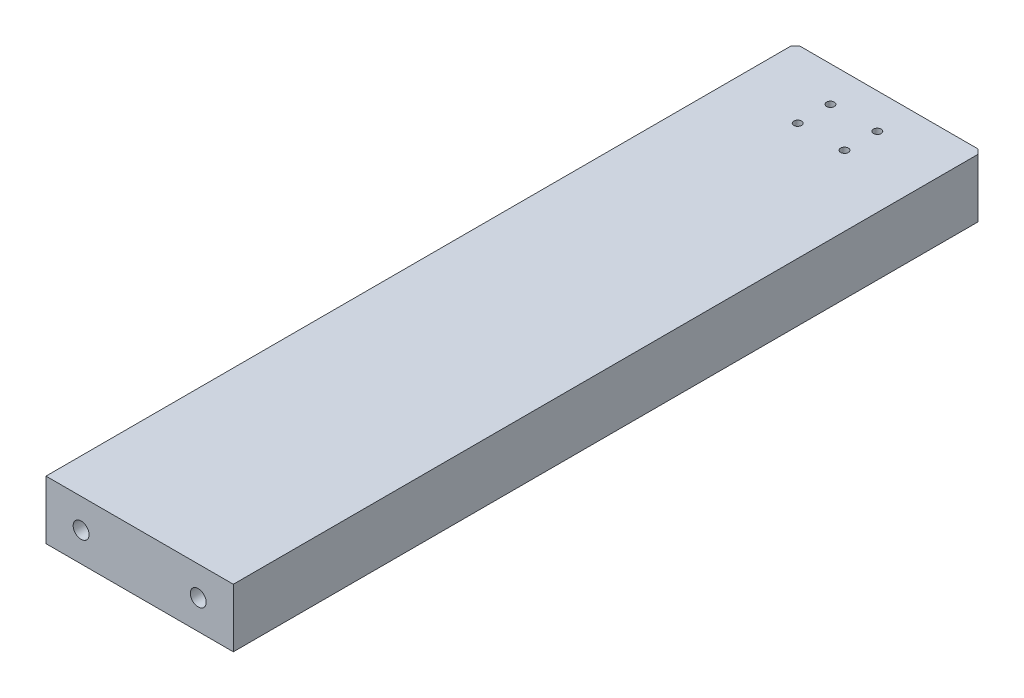
from build123d import *

# Parameters (mm, degrees)
SKETCH1_W             = 80
SKETCH1_H             = 320
BOSS_EXTRUDE1_DEPTH   = 12.5
M8_TAPPED_HOLE1_D     = 6.8
M8_TAPPED_HOLE1_DEPTH = 19.75
M8_TAPPED_HOLE1_TIP   = 2.042926105
CHAMFER1_SIZE         = 2
M4_TAPPED_HOLE1_D     = 3.3
M4_TAPPED_HOLE1_DEPTH = 10.1
M4_TAPPED_HOLE1_TIP   = 0.991420021
M8_TAPPED_HOLE2_D     = 6.8
M8_TAPPED_HOLE2_DEPTH = 19.75
M8_TAPPED_HOLE2_TIP   = 2.042926105
CUT_EXTRUDE2_DEPTH    = 15


with BuildPart() as part:
    # Sketch1 → Boss-Extrude1 (new, symmetric)
    with BuildSketch(Plane(origin=(0, 0, 0), x_dir=(1, 0, 0), z_dir=(0, 1, 0))):
        with Locations((40, 160)):
            Rectangle(SKETCH1_W, SKETCH1_H)
    extrude(amount=BOSS_EXTRUDE1_DEPTH, both=True)

    # M8 Tapped Hole1
    with Locations(Plane.XY):
        with Locations((15, 0), (65, 0)):
            Hole(M8_TAPPED_HOLE1_D / 2, depth=M8_TAPPED_HOLE1_DEPTH)
            with Locations((0, 0, -(M8_TAPPED_HOLE1_DEPTH + M8_TAPPED_HOLE1_TIP / 2))):  # 118° drill point
                Cone(0, M8_TAPPED_HOLE1_D / 2, M8_TAPPED_HOLE1_TIP, mode=Mode.SUBTRACT)

    # Chamfer1
    chamfer1_edges = [part.edges().sort_by_distance(p)[0] for p in [
        (0, 0, -320),
        (80, 0, -320),
    ]]
    chamfer(chamfer1_edges, length=CHAMFER1_SIZE)

    # M4 Tapped Hole1
    with Locations(Plane(origin=(0, 12.5, 0), x_dir=(1, 0, 0), z_dir=(0, 1, 0))):
        with Locations((30, 305), (30, 291), (50, 291), (50, 305)):
            Hole(M4_TAPPED_HOLE1_D / 2, depth=M4_TAPPED_HOLE1_DEPTH)
            with Locations((0, 0, -(M4_TAPPED_HOLE1_DEPTH + M4_TAPPED_HOLE1_TIP / 2))):  # 118° drill point
                Cone(0, M4_TAPPED_HOLE1_D / 2, M4_TAPPED_HOLE1_TIP, mode=Mode.SUBTRACT)

    # M8 Tapped Hole2
    with Locations(Plane(origin=(0, 0, -320), x_dir=(-1, 0, 0), z_dir=(0, 0, -1))):
        with Locations((-15, 0), (-65, 0)):
            Hole(M8_TAPPED_HOLE2_D / 2, depth=M8_TAPPED_HOLE2_DEPTH)
            with Locations((0, 0, -(M8_TAPPED_HOLE2_DEPTH + M8_TAPPED_HOLE2_TIP / 2))):  # 118° drill point
                Cone(0, M8_TAPPED_HOLE2_D / 2, M8_TAPPED_HOLE2_TIP, mode=Mode.SUBTRACT)

    # Sketch11 → Cut-Extrude2 (cut)
    with BuildSketch(Plane.XZ.offset(12.5)):
        with BuildLine():
            Line((50.25, -160), (50.25, -320))
            ThreePointArc((50.25, -320), (40, -330.25), (29.75, -320))
            Line((29.75, -320), (29.75, -160))
            ThreePointArc((29.75, -160), (40, -149.75), (50.25, -160))
        make_face()
    extrude(amount=-CUT_EXTRUDE2_DEPTH, mode=Mode.SUBTRACT)


solid = part.part
